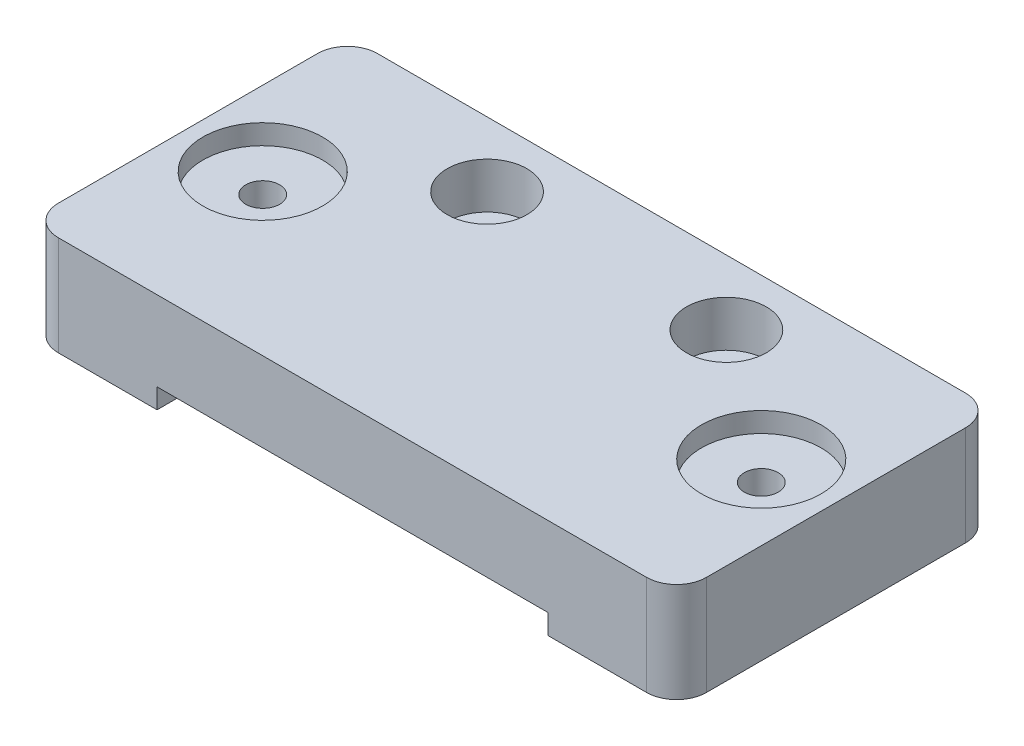
SolidWorks part; units mm, degrees
material "6061铝"
ref_plane "前视基准面" through (0, 0, 0) normal (0, 0, 1) x (1, 0, 0)
ref_plane "上视基准面" through (0, 0, 0) normal (0, 1, 0) x (1, 0, 0)
ref_plane "右视基准面" through (0, 0, 0) normal (1, 0, 0) x (0, 0, -1)
sketch "草图1" plane through (0, 0, 0) normal (0, 0, 1) x (1, 0, 0)
  line L1 (-32.5, 5) -> (32.5, 5)
  line L2 (-32.5, 5) -> (-32.5, -5)
  line L3 (-32.5, -5) -> (32.5, -5)
  line L4 (32.5, 5) -> (32.5, -5)
  line L5 (-32.5, 5) -> (32.5, -5) construction
  line L6 (-32.5, -5) -> (32.5, 5) construction
  point P0 (0, 0)
  dimension "D1" = 65
  dimension "D2" = 10
extrude "凸台-拉伸1" add sketch "草图1" along normal blind 32
hole_wizard "Ø5.0 (5) 直径孔1" positions "草图3" profile "草图4" hole size "Ø5.0" standard "GB" end condition through all
sketch "草图3" plane through (0, -5, 0) normal (0, 1, 0) x (1, 0, 0)
  line L0 (0, 0) -> (0, -27.2499) construction
  line L6 (32.5, -32) -> (-32.5, -32) construction
  point P0 (-12, -6.5)
  point P2 (12, -6.5)
  dimension "D1" = 24
  dimension "D2" = 25.5
sketch "草图4" plane through (-12, -5, 6.5) normal (1, 0, 0) x (0, 0, -1)
  line L0 (0, 0) -> (0, 10)
  line L1 (0, 10) -> (2.15, 10)
  line L2 (2.15, 10) -> (2.15, 0)
  line L5 (2.15, 0) -> (0, 0)
  line L11 (0, -6.35) -> (0, 107.95) construction
  dimension "通孔孔直径" = 4.3
  dimension "通孔孔深度" = 10
fillet "圆角1" radius 3 4 edges at (-32.5, 0, 0) (-32.5, 0, 32) (32.5, 0, 0) (32.5, 0, 32)
sketch "草图9" plane through (0, -5, 0) normal (0, -1, 0) x (1, 0, 0)
  line L1 (-19.6, -42.2127) -> (19.6, -42.2127)
  line L2 (-19.6, -42.2127) -> (-19.6, 42.2127)
  line L3 (-19.6, 42.2127) -> (19.6, 42.2127)
  line L4 (19.6, -42.2127) -> (19.6, 42.2127)
  line L5 (-19.6, -42.2127) -> (19.6, 42.2127) construction
  line L6 (-19.6, 42.2127) -> (19.6, -42.2127) construction
  point P0 (0, 0)
  dimension "D1" = 39.2
extrude "切除-拉伸2" [suppressed] cut sketch "草图9" against normal blind 2
sketch "草图10" plane through (0, 5, 0) normal (0, 1, 0) x (1, 0, 0)
  line L0 (-32.5, -16) -> (32.5, -16) construction
  line L1 (-32.5, -29) -> (-32.5, -3) construction
  line L2 (32.5, -29) -> (32.5, -3) construction
  line L3 (32.5, -16) -> (40.7581, -15.0916) construction
  line L4 (0, 0) -> (0, -42.5867) construction
  circle A0 centre (-25, -16) radius 6
  circle A1 centre (25, -16) radius 6
  dimension "D2" = 12
  dimension "D1" = 50
extrude "切除-拉伸3" cut sketch "草图10" against normal blind 2
hole_wizard "打孔尺寸(%根据)开槽圆柱头螺钉的类型1" positions "草图11" profile "草图13" counterbore size "M3" standard "GB" end condition through all
sketch "草图11" plane through (0, -5, 0) normal (0, -1, 0) x (-1, 0, 0)
  point P0 (-25, -16)
  point P3 (25, -16)
sketch "草图13" plane through (25, -5, 16) normal (1, 0, 0) x (0, 0, -1)
  line L0 (0, 0) -> (0, 10)
  line L1 (0, 10) -> (1.7, 10)
  line L3 (1.7, 10) -> (1.7, 3.4)
  line L4 (1.7, 3.4) -> (3, 3.4)
  line L5 (3, 3.4) -> (3, 0)
  line L7 (3, 0) -> (0, 0)
  line L11 (0, -6.35) -> (0, 107.95) construction
  dimension "通孔孔直径" = 3.4
  dimension "通孔孔深度" = 10
  dimension "柱形沉头孔直径" = 6
  dimension "柱形沉头孔深度" = 3.4
hole_wizard "打孔尺寸(%根据)开槽圆柱头螺钉的类型2" positions "草图14" profile "草图15" counterbore size "M4" standard "GB" end condition through all
sketch "草图14" plane through (0, 5, 0) normal (0, 1, 0) x (1, 0, 0)
  point P0 (-12, -6.5)
  point P3 (12, -6.5)
sketch "草图15" plane through (-12, 5, 6.5) normal (1, 0, 0) x (0, 0, 1)
  line L0 (0, 0) -> (0, 10)
  line L1 (0, 10) -> (2.15, 10)
  line L3 (2.15, 10) -> (2.15, 4.6)
  line L4 (2.15, 4.6) -> (4, 4.6)
  line L5 (4, 4.6) -> (4, 0)
  line L7 (4, 0) -> (0, 0)
  line L11 (0, -6.35) -> (0, 107.95) construction
  dimension "通孔孔直径" = 4.3
  dimension "通孔孔深度" = 10
  dimension "柱形沉头孔直径" = 8
  dimension "柱形沉头孔深度" = 4.6
sketch "草图16" plane through (0, -5, 0) normal (0, -1, 0) x (1, 0, 0)
  line L1 (-19.6, -36.4419) -> (19.6, -36.4419)
  line L2 (-19.6, -36.4419) -> (-19.6, 36.4419)
  line L3 (-19.6, 36.4419) -> (19.6, 36.4419)
  line L4 (19.6, -36.4419) -> (19.6, 36.4419)
  line L5 (-19.6, -36.4419) -> (19.6, 36.4419) construction
  line L6 (-19.6, 36.4419) -> (19.6, -36.4419) construction
  point P0 (0, 0)
  dimension "D1" = 39.2
extrude "切除-拉伸4" cut sketch "草图16" against normal blind 2
